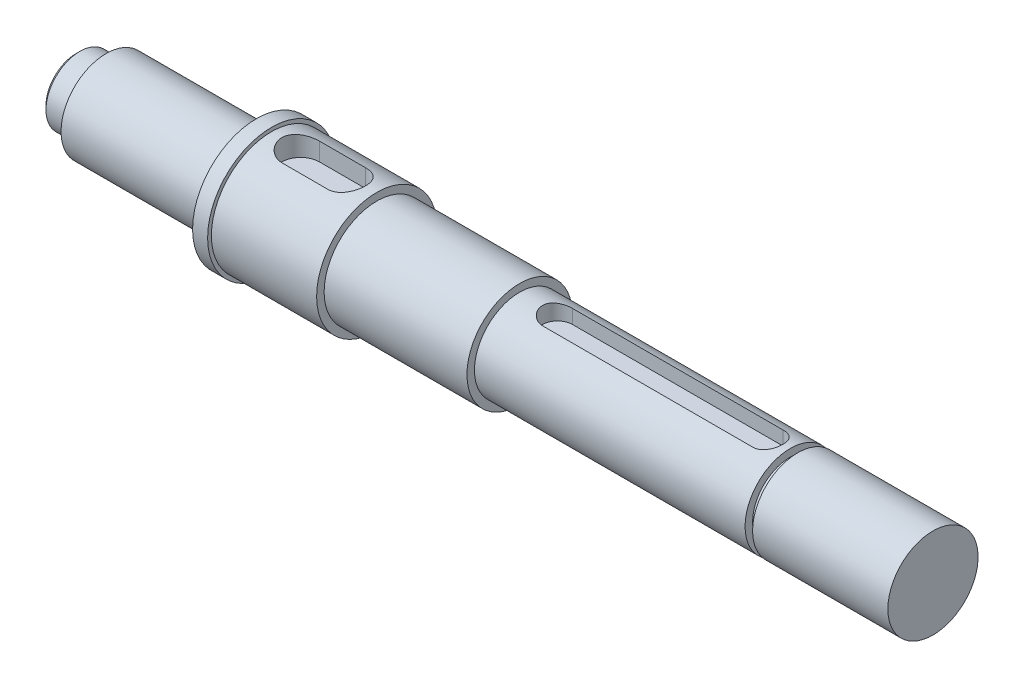
SolidWorks part; units mm, degrees
ref_plane "前视基准面" through (0, 0, 0) normal (0, 0, 1) x (1, 0, 0)
ref_plane "上视基准面" through (0, 0, 0) normal (0, 1, 0) x (1, 0, 0)
ref_plane "右视基准面" through (0, 0, 0) normal (1, 0, 0) x (0, 0, -1)
other "Configuration Table"
sketch "草图1" plane through (0, 0, 0) normal (0, 0, 1) x (1, 0, 0)
  line L0 (-80.0849, 0) -> (91.7912, 0) construction
  line L20 (-46.1039, 8.5) -> (-44.1039, 8.5)
  line L21 (-69.6039, 4.5) -> (-66.1039, 4.5)
  line L22 (-70.1039, 4) -> (-70.1039, 0)
  line L23 (-66.1039, 4.5) -> (-66.1039, 6)
  line L24 (-46.1039, 6) -> (-66.1039, 6)
  line L25 (-46.1039, 6) -> (-46.1039, 8.5)
  line L26 (-44.1039, 8.5) -> (-44.1039, 8)
  line L27 (-44.1039, 8) -> (-30.1039, 8)
  line L28 (-30.1039, 8) -> (-30.1039, 7)
  line L29 (-30.1039, 7) -> (-11.1039, 7)
  line L30 (-11.1039, 7) -> (-11.1039, 6)
  line L31 (-11.1039, 6) -> (24.8961, 6)
  line L32 (24.8961, 6) -> (24.8961, 5)
  line L33 (24.8961, 5) -> (25.8961, 5)
  line L34 (25.8961, 5) -> (25.8961, 6)
  line L35 (25.8961, 6) -> (43.8961, 6)
  line L36 (43.8961, 6) -> (43.8961, 0)
  line L37 (-70.1039, 4) -> (-69.6039, 4.5)
  line L38 (-70.1039, 0) -> (43.8961, 0)
  point P28 (-70.1039, 4.5)
  dimension "D3" = 0
  dimension "D4" = 4
  dimension "D13" = 4
  dimension "D14" = 14
  dimension "D15" = 19
  dimension "D16" = 36
  dimension "D17" = 18
  dimension "D18" = 1
  dimension "D19" = 1
  dimension "D20" = 1
  dimension "D21" = 2
  dimension "D22" = 20
  dimension "D23" = 0.5
  dimension "D24" = 0.5
revolve "旋转1" add sketch "草图1" angle 360 about L38
cosmetic thread "装饰螺纹线1" parameters "D2"=11
ref_plane "基准面3" through (0, 6, 0) normal (0, 1, 0) x (1, 0, 0)
sketch "草图7" plane through (0, 6, 0) normal (0, 1, 0) x (1, 0, 0)
  line L0 (-9.8969, 0) -> (22.7069, 0) construction
  line L1 (-6.0539, 0) -> (21.9461, 0) construction
  line L2 (-6.0539, 2) -> (21.9461, 2)
  line L3 (-6.0539, -2) -> (21.9461, -2)
  line L6 (24.8961, -5) -> (24.8961, 5) construction
  arc A0 (-6.0539, 2) -> (-6.0539, -2) centre (-6.0539, 0) ccw
  arc A1 (21.9461, -2) -> (21.9461, 2) centre (21.9461, 0) ccw
  point P5 (7.9461, 0)
  dimension "D1" = 28
  dimension "D2" = 2
  dimension "D3" = 2.95
extrude "切除-拉伸1" cut sketch "草图7" against normal blind 2.2
ref_plane "基准面4" through (0, 8, 0) normal (0, 1, 0) x (1, 0, 0)
sketch "草图9" plane through (0, 8, 0) normal (0, 1, 0) x (1, 0, 0)
  line L0 (-50.8196, 0) -> (0, 0) construction
  line L1 (-40.2254, 0) -> (-34.1039, 0) construction
  line L2 (-40.2254, 2.5) -> (-34.1039, 2.5)
  line L3 (-40.2254, -2.5) -> (-34.1039, -2.5)
  line L4 (-44.1039, -8) -> (-44.1039, 8) construction
  arc A0 (-40.2254, 2.5) -> (-40.2254, -2.5) centre (-40.2254, 0) ccw
  arc A1 (-34.1039, -2.5) -> (-34.1039, 2.5) centre (-34.1039, 0) ccw
  point P5 (-37.1646, 0)
  dimension "D1" = 10
  dimension "D3" = 2.5
  dimension "D2" = 6.1214
extrude "切除-拉伸2" cut sketch "草图9" against normal blind 2.8
